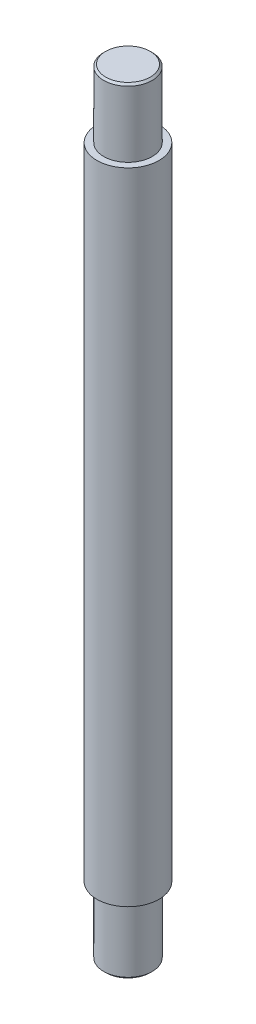
from build123d import *

# Parameters (mm, degrees)
CHAMFER1_SIZE = 1


with BuildPart() as part:
    # Sketch1 → Revolve1 (revolve)
    with BuildSketch(Plane.XY, mode=Mode.PRIVATE) as revolve1_sk:
        Polygon((0, 0), (12.5, 0), (12.5, 35), (16, 35), (16, 365), (12.5, 365), (12.5, 400), (0, 400), align=None)
    revolve(revolve1_sk.sketch.rotate(Axis((0, 400, 0), (0, -1, 0)), 180), axis=Axis((0, 400, 0), (0, -1, 0)))

    # Chamfer1
    chamfer1_edges = [part.edges().sort_by_distance(p)[0] for p in [
        (12.5, 400, 0),
        (12.5, 0, 0),
    ]]
    chamfer(chamfer1_edges, length=CHAMFER1_SIZE)


solid = part.part
